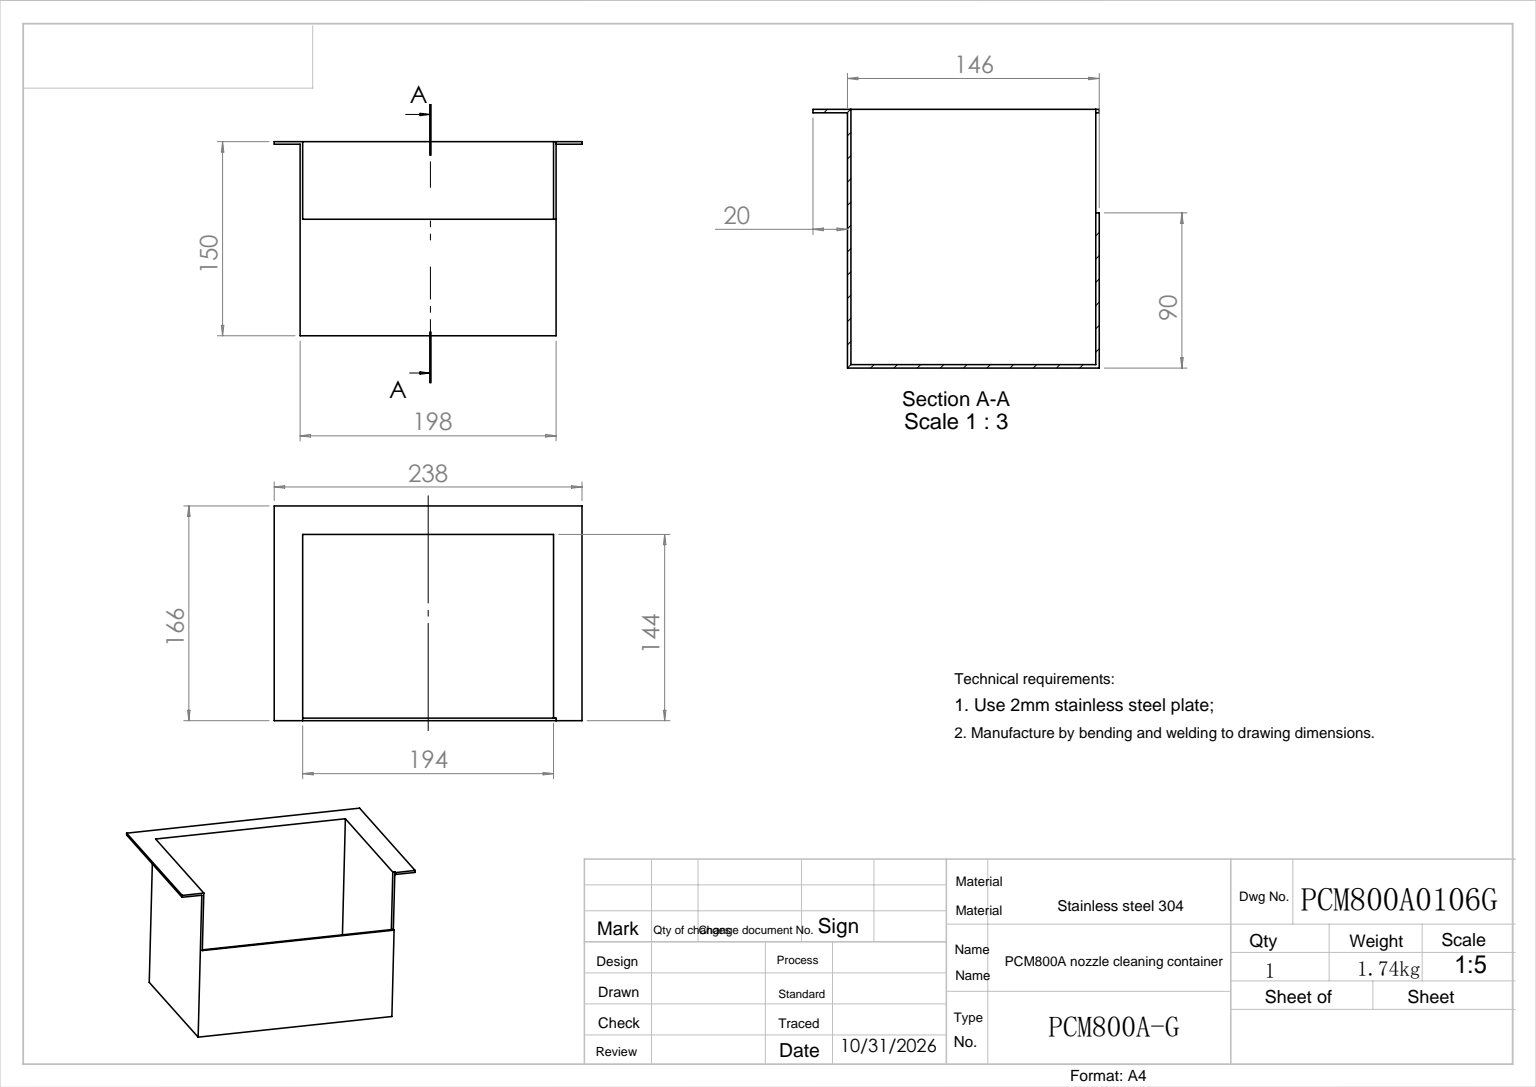
SolidWorks part; units mm, degrees
ref_plane "前视基准面" through (0, 0, 0) normal (0, 0, 1) x (1, 0, 0)
ref_plane "上视基准面" through (0, 0, 0) normal (0, 1, 0) x (1, 0, 0)
ref_plane "右视基准面" through (0, 0, 0) normal (1, 0, 0) x (0, 0, -1)
sketch "草图1" plane through (0, 0, 0) normal (0, 0, 1) x (1, 0, 0)
  line L1 (0, 0) -> (198, 0)
  line L2 (0, 0) -> (0, -146)
  line L3 (0, -146) -> (198, -146)
  line L4 (198, 0) -> (198, -146)
  dimension "D1" = 198
  dimension "D2" = 146
extrude "凸台-拉伸1" add sketch "草图1" along normal blind 150
shell "抽壳1" thickness 2
sketch "草图2" plane through (0, 0, 150) normal (0, 0, 1) x (1, 0, 0)
  line L0 (198, 0) -> (0, 0) construction
  line L1 (0, 0) -> (0, -146) construction
  line L2 (198, -146) -> (198, 0) construction
  line L3 (0, -146) -> (-20, -146)
  line L4 (198, 0) -> (0, 0)
  line L5 (0, 0) -> (0, -146)
  line L6 (198, -146) -> (198, 0)
  line L7 (198, -146) -> (218, -146)
  line L8 (218, 20) -> (-20, 20)
  line L9 (-20, 20) -> (-20, -146)
  line L11 (218, -146) -> (218, 20)
  line L12 (0, -146) -> (198, -146) construction
  line L13 (-20, -166) -> (218, -166) construction
  line L14 (218, -166) -> (218, 20) construction
  line L15 (-20, 20) -> (-20, -166) construction
  dimension "D1" = 20
extrude "凸台-拉伸2" add sketch "草图2" against normal blind 2
sketch "草图3" plane through (0, -146, 0) normal (0, -1, 0) x (1, 0, 0)
  line L0 (-20, 150) -> (218, 150) construction
  line L1 (2, 150) -> (198, 150)
  line L2 (2, 150) -> (2, 90)
  line L3 (2, 90) -> (198, 90)
  line L4 (198, 150) -> (198, 90)
  line L5 (0, 148) -> (0, 0) construction
  dimension "D1" = 196
  dimension "D2" = 2
  dimension "D3" = 60
extrude "切除-拉伸1" cut sketch "草图3" against normal blind 2
